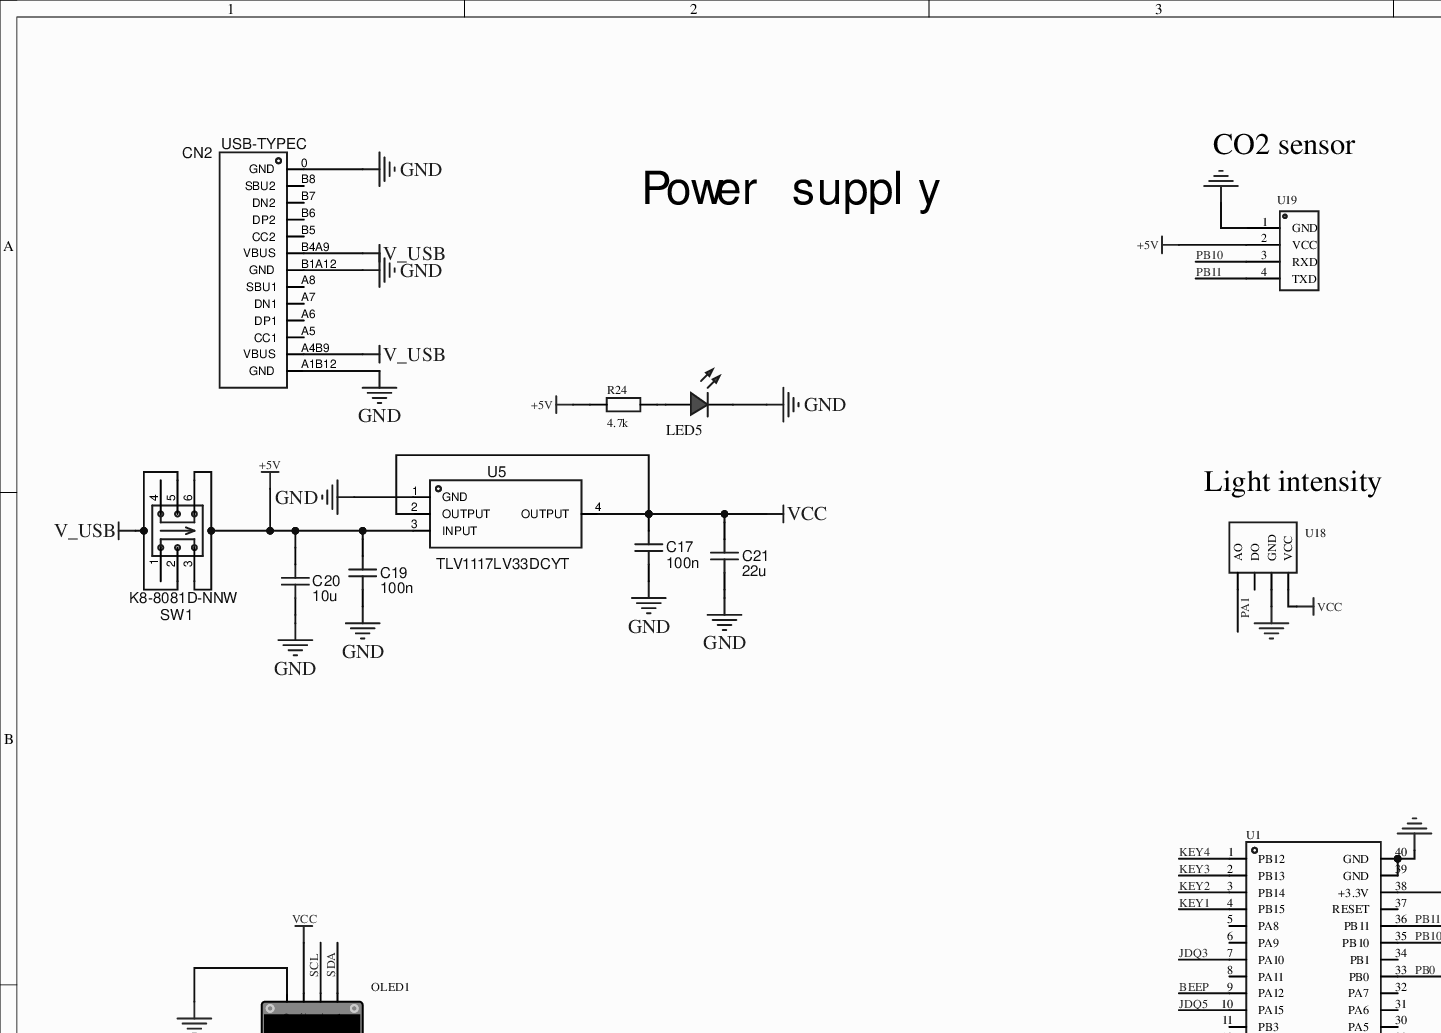
[diagram p0: MISC51965-3.schdoc, top left]
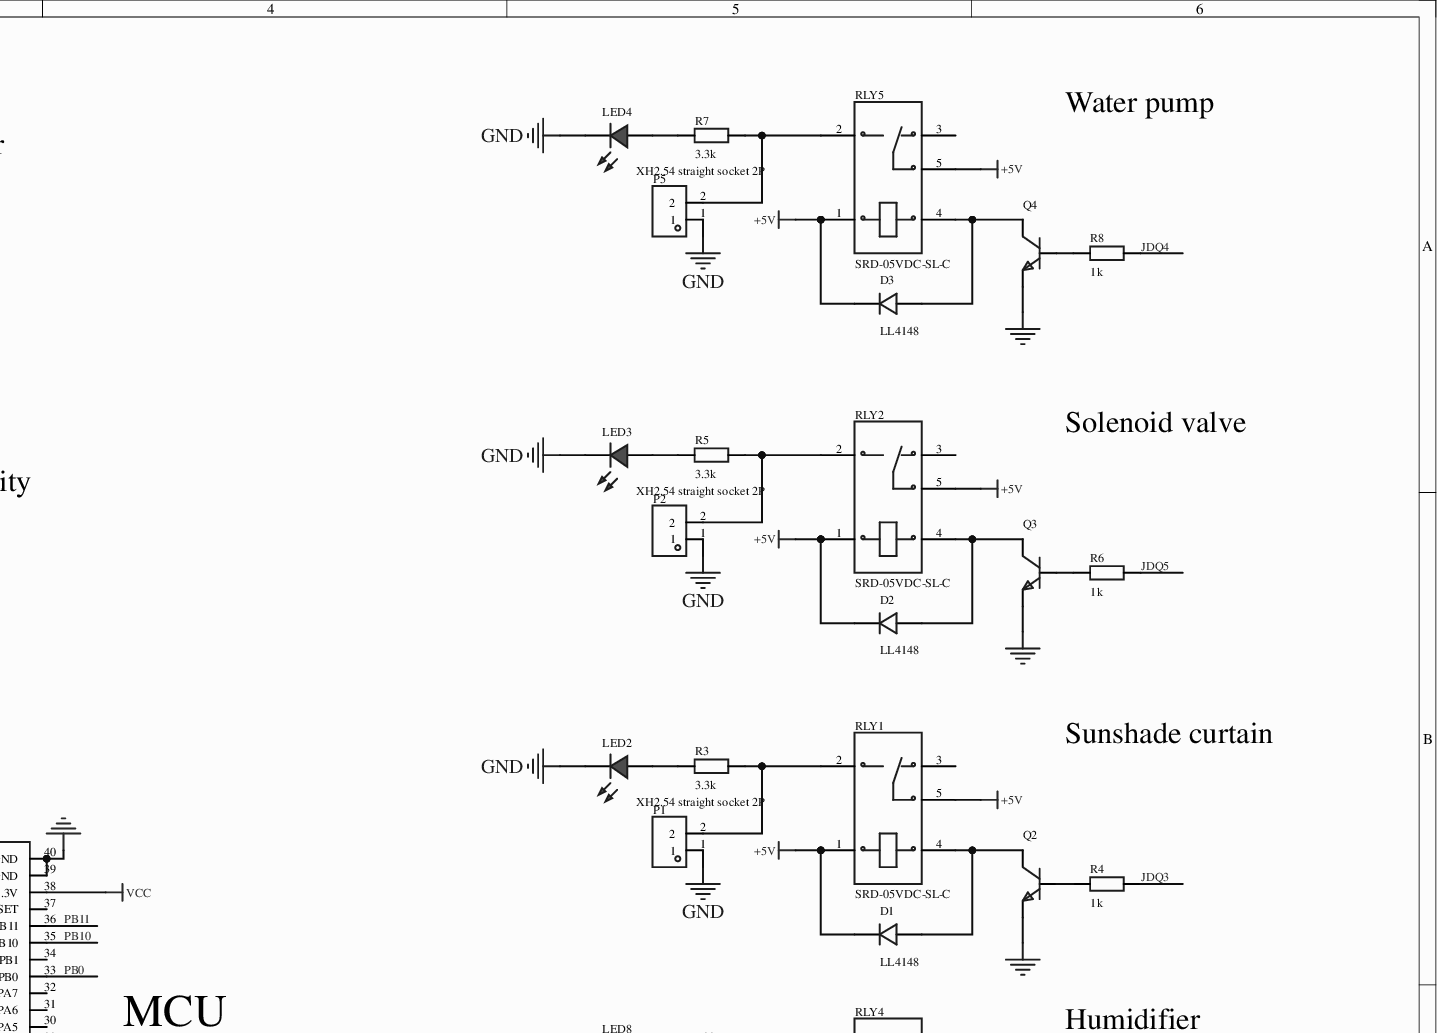
[diagram p1: MISC51965-3.schdoc, top right]
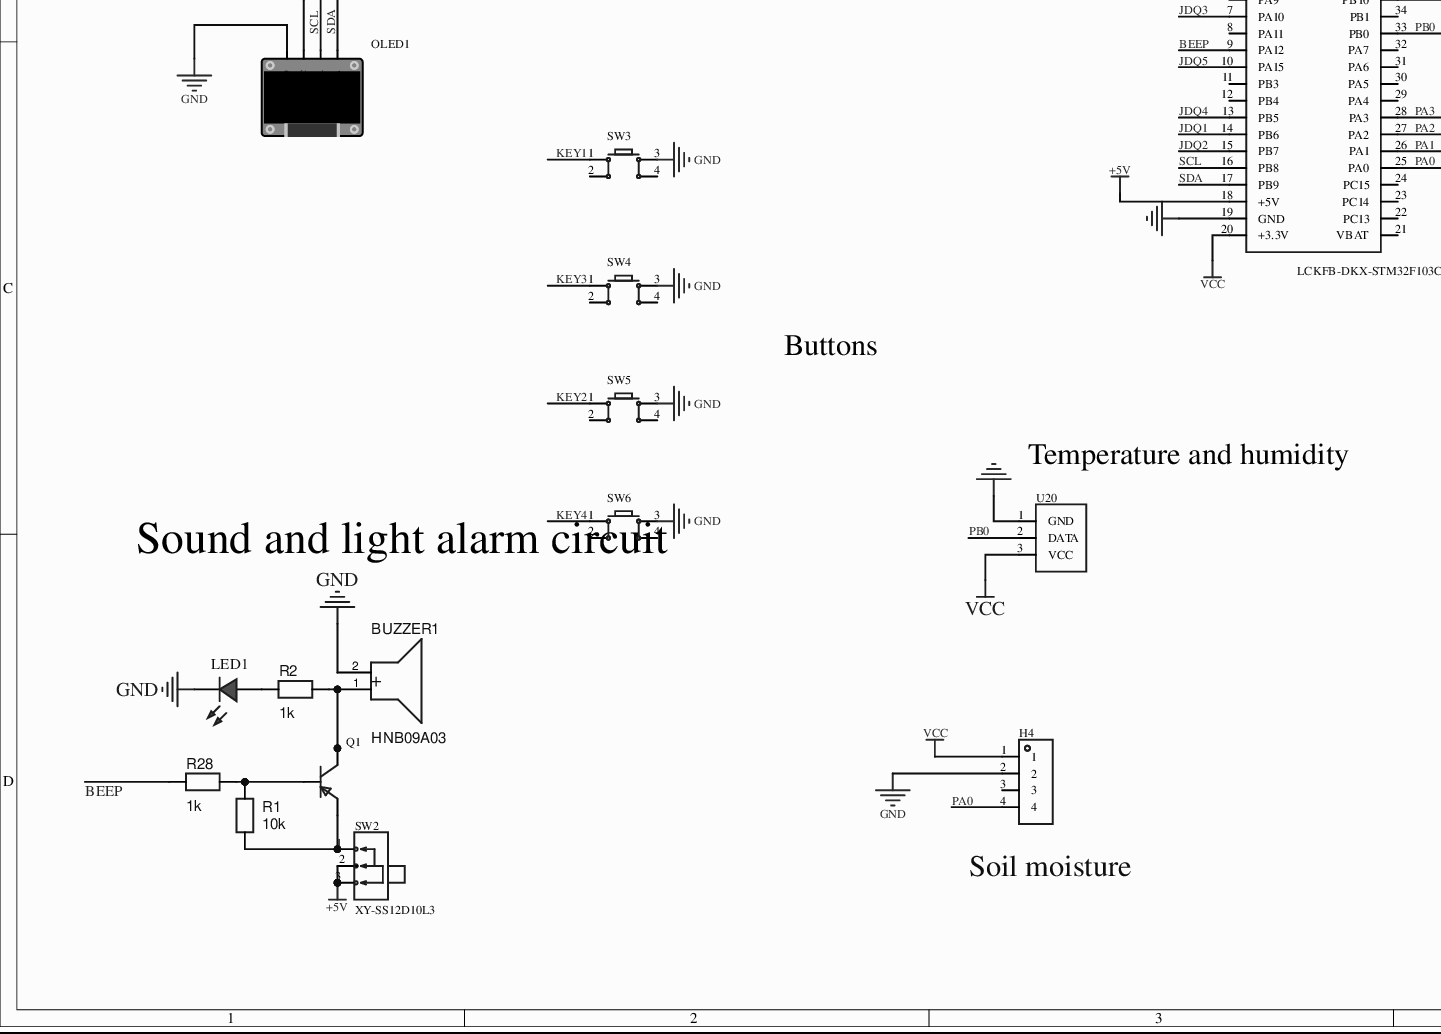
[diagram p2: MISC51965-3.schdoc, bottom left]
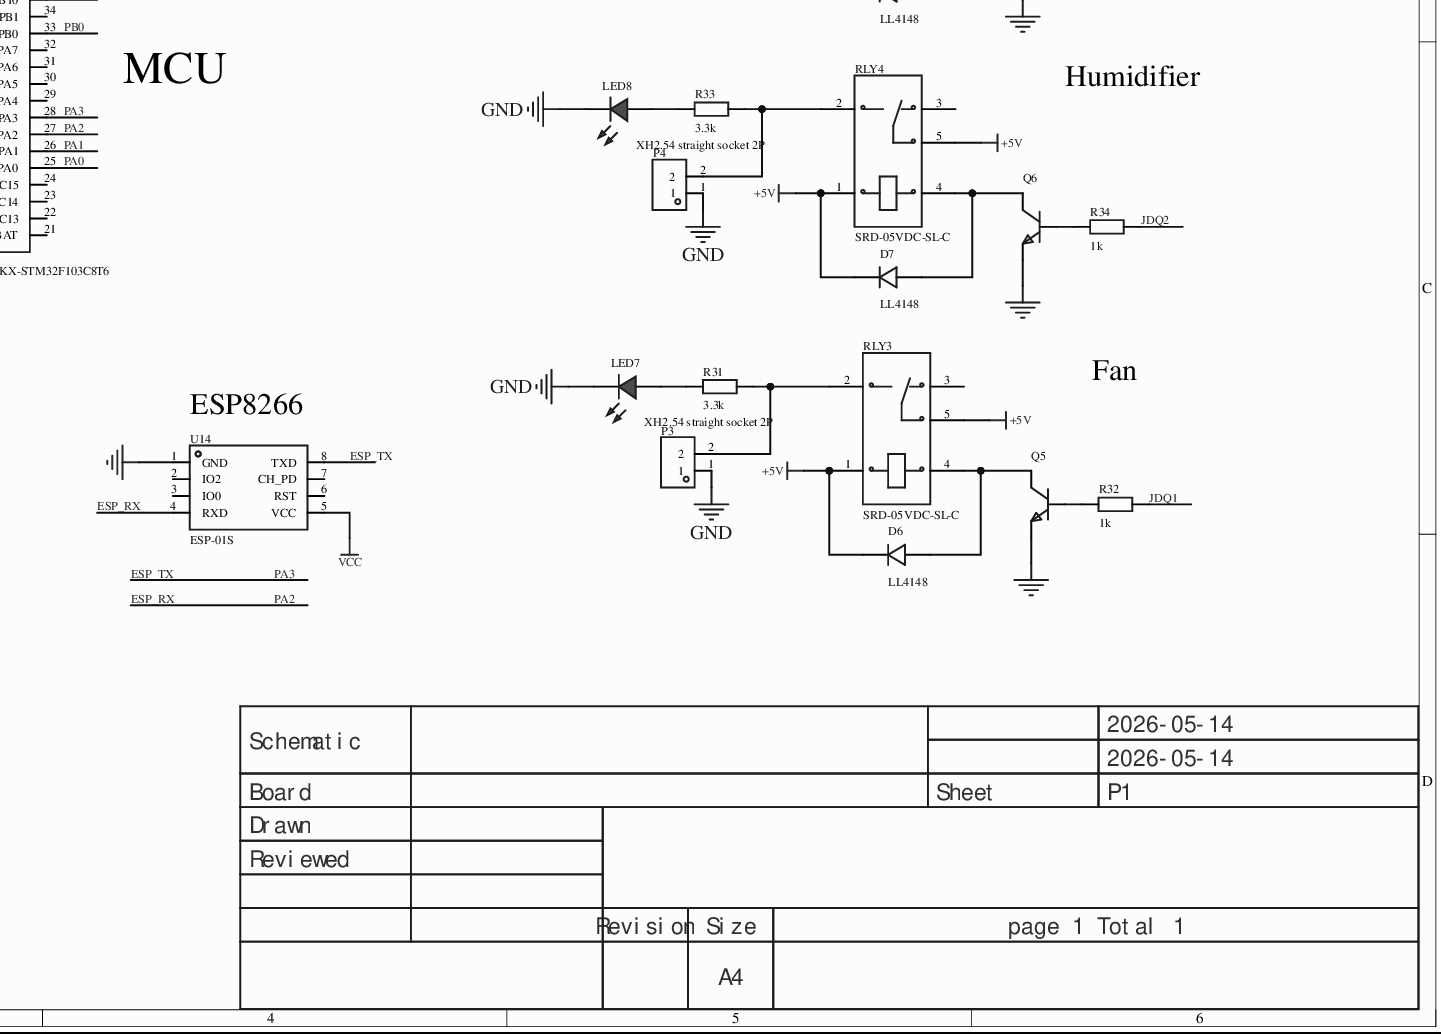
[diagram p3: MISC51965-3.schdoc, bottom right]
# Altium project MISC51965-2.PrjPcb
1 sheet, 62 parts. Net scope: global (net labels, ports and power ports of the same name join across sheets).
Board file: MISC51965.pcbdoc

## Sheet MISC51965-3.schdoc
size 420 x 297 mm; Version: V1.0; @Project Name: MISC51965; @Update Date: 2026-05-14; @Create Date: 2026-05-14; @Board Name: MISC51965; @Create Time: 12:43:51; @Page Count: 1; @Page No: 1; @Schematic Name: MISC51965; @Update Time: 12:43:51; Size: A4

### Parts
BUZZER1  HNB09A03  [BUZ-TH_BD9.0-P5.00-D0.6-FD]
C17  100n  [C0603]
C19  100n  [C0603]
C20  10u  [C0603]
C21  22u  [C0603]
CN2  USB-TYPEC  [USB-C-SMD_MC-307]
D1  LL4148  [LL-34_L3.5-W1.5-RD]
D2  LL4148  [LL-34_L3.5-W1.5-RD]
D3  LL4148  [LL-34_L3.5-W1.5-RD]
D6  LL4148  [LL-34_L3.5-W1.5-RD]
D7  LL4148  [LL-34_L3.5-W1.5-RD]
H4  (no value)  [HDR-TH_4P-P2.54-V-F]
LED1  (no value)  [LED_0603]
LED2  (no value)  [LED_TH-3mm]
LED3  (no value)  [LED_TH-3mm]
LED4  (no value)  [LED_TH-3mm]
LED5  (no value)  [LED_0603]
LED7  (no value)  [LED_TH-3mm]
LED8  (no value)  [LED_TH-3mm]
OLED1  (no value)  [0.96OLED_4P]
P1  XH2.54 straight socket 2P  [CONN-TH_XH2.54-2P]
P2  XH2.54 straight socket 2P  [CONN-TH_XH2.54-2P]
P3  XH2.54 straight socket 2P  [CONN-TH_XH2.54-2P]
P4  XH2.54 straight socket 2P  [CONN-TH_XH2.54-2P]
P5  XH2.54 straight socket 2P  [CONN-TH_XH2.54-2P]
Q1  (no value)  [S8550P_SOT]
Q2  (no value)  [S8050_SOT-23]
Q3  (no value)  [S8050_SOT-23]
Q4  (no value)  [S8050_SOT-23]
Q5  (no value)  [S8050_SOT-23]
Q6  (no value)  [S8050_SOT-23]
R1  10k  [R0603]
R2  1k  [R0603]
R3  3.3k  [R0603]
R4  1k  [R0603]
R5  3.3k  [R0603]
R6  1k  [R0603]
R7  3.3k  [R0603]
R8  1k  [R0603]
R24  4.7k  [R0805]
R28  1k  [R0603]
R31  3.3k  [R0603]
R32  1k  [R0603]
R33  3.3k  [R0603]
R34  1k  [R0603]
RLY1  SRD-05VDC-SL-C  [RELAY-TH_SRD-XXVDC-XL-C]
RLY2  SRD-05VDC-SL-C  [RELAY-TH_SRD-XXVDC-XL-C]
RLY3  SRD-05VDC-SL-C  [RELAY-TH_SRD-XXVDC-XL-C]
RLY4  SRD-05VDC-SL-C  [RELAY-TH_SRD-XXVDC-XL-C]
RLY5  SRD-05VDC-SL-C  [RELAY-TH_SRD-XXVDC-XL-C]
SW1  K8-8081D-NNW  [SW-TH_6P-L8.0-W8.0-P2.50]
SW2  XY-SS12D10L3  [SW-TH_3P-L12.7-W6.7_XY-SS12D10LXX]
SW3  (no value)  [SW-TH_4P-L6.0-W6.0-P4.50-LS6.5]
SW4  (no value)  [SW-TH_4P-L6.0-W6.0-P4.50-LS6.5]
SW5  (no value)  [SW-TH_4P-L6.0-W6.0-P4.50-LS6.5]
SW6  (no value)  [SW-TH_4P-L6.0-W6.0-P4.50-LS6.5]
U1  LCKFB-DKX-STM32F103C8T6  [CONN-TH_L53.3-W22.9_STM32F103C8T6-CARD]
U5  TLV1117LV33DCYT  [SOT-223-4_L6.5-W3.5-P2.30-LS7.0-BR]
U14  ESP-01S  [WIFIM-TH_ESP-01S]
U18  Light intensity module  [光敏传感器]  (value not drawn)
U19  (no value)  [4P排母]
U20  (no value)  [dht11温湿度传感器]

### Nets
+5V: C19.2 C20.2 D1.1(K) D2.1(K) D3.1(K) D6.1(K) D7.1(K) R24.1 RLY1.1 RLY1.5 RLY2.1 RLY2.5 RLY3.1 RLY3.5 RLY4.1 RLY4.5 RLY5.1 RLY5.5 SW1.3 SW1.6 SW2.2 SW2.3 U1.18(+5V) U5.3(INPUT) U19.2(VCC)
GND: BUZZER1.2(-) C17.1 C19.1 C20.1 C21.1 CN2.0(GND) CN2.A1B12(GND) CN2.B1A12(GND) H4.2 LED1.1(C) LED2.2(A) LED3.2(A) LED4.2(A) LED5.1(C) LED7.2(A) LED8.2(A) OLED1.1(GND) P1.1 P2.1 P3.1 P4.1 P5.1 Q2.2 Q3.2 Q4.2 Q5.2 Q6.2 SW3.3 SW4.3 SW5.3 SW6.3 U1.19(GND) U1.39(GND) U1.40(GND) U5.1(GND) U14.1(GND) U18.2(GND) U19.1(GND) U20.1(GND)
V_USB: CN2.A4B9(VBUS) CN2.B4A9(VBUS) SW1.2 SW1.5
VCC: C17.2 C21.2 H4.1 OLED1.2(VCC) U1.20(+3.3V) U1.38(+3.3V) U5.2(OUTPUT) U5.4(OUTPUT) U14.5(VCC) U18.1(VCC) U20.3(VCC)
BEEP: R28.1 U1.9(PA12)
ESP_RX: U1.27(PA2) U14.4(RXD)  [also labelled PA2]
ESP_TX: U1.28(PA3) U14.8(TXD)  [also labelled PA3]
JDQ1: R32.1 U1.14(PB6)
JDQ2: R34.1 U1.15(PB7)
JDQ3: R4.1 U1.7(PA10)
JDQ4: R8.1 U1.13(PB5)
JDQ5: R6.1 U1.10(PA15)
KEY1: SW3.1 U1.4(PB15)
KEY2: SW5.1 U1.3(PB14)
KEY3: SW4.1 U1.2(PB13)
KEY4: SW6.1 U1.1(PB12)
PA0: H4.4 U1.25(PA0)
PA1: U1.26(PA1) U18.4(AO)
PB0: U1.33(PB0) U20.2(DATA)
PB10: U1.35(PB10) U19.3(RXD)
PB11: U1.36(PB11) U19.4(TXD)
SCL: OLED1.3(SCL) U1.16(PB8)
SDA: OLED1.4(SDA) U1.17(PB9)
NetBUZZER1_1: BUZZER1.1(+) Q1.3(C) R2.2
NetD1_2: D1.2(A) Q2.3 RLY1.4
NetD2_2: D2.2(A) Q3.3 RLY2.4
NetD3_2: D3.2(A) Q4.3 RLY5.4
NetD6_2: D6.2(A) Q5.3 RLY3.4
NetD7_2: D7.2(A) Q6.3 RLY4.4
NetLED1_2: LED1.2(A) R2.1
NetLED2_1: LED2.1(C) R3.2
NetLED3_1: LED3.1(C) R5.2
NetLED4_1: LED4.1(C) R7.2
NetLED5_2: LED5.2(A) R24.2
NetLED7_1: LED7.1(C) R31.2
NetLED8_1: LED8.1(C) R33.2
NetP1_2: P1.2 R3.1 RLY1.2
NetP2_2: P2.2 R5.1 RLY2.2
NetP3_2: P3.2 R31.1 RLY3.2
NetP4_2: P4.2 R33.1 RLY4.2
NetP5_2: P5.2 R7.1 RLY5.2
NetQ1_1: Q1.1(B) R1.2 R28.2
NetQ1_2: Q1.2(E) R1.1 SW2.1
NetQ2_1: Q2.1 R4.2
NetQ3_1: Q3.1 R6.2
NetQ4_1: Q4.1 R8.2
NetQ5_1: Q5.1 R32.2
NetQ6_1: Q6.1 R34.2

Not connected (* = marked no-connect by the designer): CN2 A5(CC1)* A6(DP1) A7(DN1) A8(SBU1)* B5(CC2)* B6(DP2) B7(DN2) B8(SBU2)*; H4 3; RLY1 3*; RLY2 3*; RLY3 3*; RLY4 3*; RLY5 3*; SW1 1* 4*; SW3 2 4; SW4 2 4; SW5 2 4; SW6 2 4; U1 5(PA8) 6(PA9) 8(PA11) 11(PB3) 12(PB4) 21(VBAT) 22(PC13) 23(PC14) 24(PC15) 29(PA4) 30(PA5) 31(PA6) 32(PA7) 34(PB1) 37(RESET); U14 2(IO2)* 3(IO0)* 6(RST)* 7(CH_PD)*; U18 3(DO)*

### Notes on the sheet
- CO2 sensor
- Water pump
- Power supply
- Light intensity
- Solenoid valve
- Sunshade curtain
- MCU
- Humidifier
- Buttons
- Fan
- (near U20) Temperature and humidity
- (near U14) ESP8266
- (near SW6) Sound and light alarm circuit
- (near H4) Soil moisture
- 2026-05-14
- Schematic
- Board
- Sheet
- P1
- Drawn
- Reviewed
- Revision
- Size
- A4
- page 1 Total 1

### Library data of the parts
BUZZER1 = HNB09A03: Manufacturer: 华能; Add into BOM: yes; Frequency: 3kHz; Symbol: HNB09A03; Device: HNB09A03; Convert to PCB: yes; Origin Footprint: BUZ-TH_BD9.0-P5.00-D0.6-FD; Supplier: LCSC; Supplier Part: C96102; Manufacturer Part: HNB09A03; JLCPCB Part Class: Extended Part; FootprintName: BUZ-TH_BD9.0-P5.00-D0.6-FD
C17 C19-C21 = 100n: Add into BOM: yes; Symbol: 100n; Device: 100n; Convert to PCB: yes; Origin Footprint: C0603; FootprintName: C0603
CN2 = MC-307: Manufacturer: HANBO(汉博); Add into BOM: yes; Symbol: USB-TYPEC; Device: MC-307; Convert to PCB: yes; Origin Footprint: USB-C-SMD_MC-307; Supplier: LCSC; Supplier Part: C961709; Manufacturer Part: MC-307; JLCPCB Part Class: Extended Part; FootprintName: USB-C-SMD_MC-307
D1-D3 D6 D7 = LL4148_C9808: Diode configuration: -; power: 500mW; DC reverse withstand voltage (Vr): 75V; average rectified current (Io): 200mA; forward voltage (Vf): 1V@10mA; reverse current (Ir): 5uA@75V; reverse recovery time (trr): 4ns; operating temperature: +175℃@(Tj);; Manufacturer: ST(先科); 3D Model: 4a6f2309ca4c4217857da1816cccdf69; 3D Model Transform: 133.93674,59.031,0,0,0,0,0,0,0; AddInBom: yes; ModelName: LL-34_L3.5-W1.5; Symbol: LL4148; Device: LL4148_C9808; LCSC Part Name: 75V 200mA 4ns; Supplier Part: C9808; Manufacturer Part: LL4148; Supplier Footprint: LL-34; JLCPCB Part Class: Basic library; Datasheet: https://example.com/upload/public/pdf/source/20121108/1457706554347.pdf; Supplier: LCSC; Diode Configuration: -; Power Dissipation: 500mW; Reverse Voltage (Vr): 75V; Average Rectified Current (Io): 200mA; Forward Voltage (Vf@If): 1V@10mA; Reverse Leakage Current: 5uA@75V; Reverse Recovery Time (trr): 4ns; Operating Temperature: +175℃@(Tj); ConvertToPcb: yes; FootprintName: LL-34_L3.5-W1.5-RD
H4 = HDR-F_2.54_1x4P: Symbol: 2.54-1*4P female; 3D Model: d187812051054f85879fcaa51a310d8e0819f05c4eef4c71ace90d822a990e87; 3D Model Transform: 419.6842,98.464,0,0,0,0,0,0,-118.11; ConvertToPcb: yes; Device: HDR-F_2.54_1x4P; Supplier Part: C2718488; Supplier Footprint: 插件; FootprintName: HDR-TH_4P-P2.54-V-F; AddInBom: yes; ModelName: HDR-TH_4P-P2.54-V-F
LED1 LED5 = LED_0603-R: Symbol: LED_R; Convert to PCB: yes; 3D Model: dd8257b0d61a4cd7b68939a056e08095; 3D Model Transform: 58.72,29.4,22.03,0,0,0,0,0,0; ModelName: LED-0603_R; Device: LED_0603-R; Add into BOM: yes; Supplier Footprint: 0603; FootprintName: LED_0603
LED2-LED4 LED7 LED8 = LED_TH-R_3mm: 3D Model: a497c992633541038a38947cdc58012f; 3D Model Transform: 141.274,153.327,0,0,0,0,-5.984,0,-137.795; ConvertToPcb: yes; ModelName: LED-TH-3mm_R; Symbol: LED_TH-R; Device: LED_TH-R_3mm; Supplier Footprint: 插件; AddInBom: yes; FootprintName: LED_TH-3mm
OLED1 = 0.96OLED模块_4P: Symbol: 0.96OLED module_4P; ConvertToPcb: yes; ModelId: 79c000fdb68d45a296c2e9bedf4f90550819f05c4eef4c71ace90d822a990e87; ModelTransform: 1393.69792,1318.895,0,0,0,0,0,-560.079,-137.795; Device: 0.96OLED module_4P; AddInBom: yes; FootprintName: 0.96OLED_4P; Supplier Footprint: 插件; ModelName: 0.96OLED_4P
P1-P5 = XH2.54直插座-2P: 3D Model: dc9654a6caad4c20aab3bc231ea458cf; 3D Model Transform: 296.889,230.315,0,0,0,0,0,26.653,-137.795; AddInBom: yes; Symbol: XH2.54 straight socket 2P; Device: XH2.54 straight socket 2P; LCSC Part Name: XH2.54直插座-2P; Supplier Part: C9900016957; Manufacturer Part: XH2.54直插座-2P; Supplier Footprint: XH2.54-2; JLCPCB Part Class: Extended library; Supplier: LCSC; ConvertToPcb: yes; FootprintName: CONN-TH_XH2.54-2P; ModelName: CONN-TH_XH2.54-2P
Q1 = S8550_SOT_PNP: Symbol: PNP; ConvertToPcb: yes; ModelId: 9c0df02d6f3e44e889da37f3e5bf54960819f05c4eef4c71ace90d822a990e87; ModelName: SOT-23-3_L2.9-W1.4-P1.90-LS2.5-BR; ModelTransform: 98.43,114.17,37.91,0,0,0,0,0,0; Device: S8550_SOT_PNP; AddInBom: yes; Supplier Footprint: SOT-23; FootprintName: S8550P_SOT
Q2-Q6 = S8050_SOT_NPN: Symbol: NPN; 3D Model: c62791f0466c4ae2a892c056b845b0ca; 3D Model Transform: 98.6,114.12,41.29,180,0,0,0,0,-3; ConvertToPcb: yes; ModelName: SOT-23-3P_L2.9-W1.3-H1.0-LS2.4-P0.95; Device: S8050_SOT_NPN; Supplier Footprint: SOT-23; AddInBom: yes; FootprintName: S8050_SOT-23
R1 R2 R28 = 1k: Add into BOM: yes; Symbol: 1k; Device: 1k; Convert to PCB: yes; Origin Footprint: R0603; FootprintName: R0603
R3-R8 R31-R34 = Res_0603: Symbol: Resistor; 3D Model: fc143cca1e79419f9cd78b61e9279f08; 3D Model Transform: 31.8897,63.7794,0,90,0,0,0,0,0; ConvertToPcb: yes; Device: Res_0603; Supplier Footprint: 0603; AddInBom: yes; FootprintName: R0603; ModelName: R0603
  R3 R5 R7 R31 R33: Value: 3.3k
  R4 R6 R8 R32 R34: Value: 1k
R24 = 0805W8F1002T5E_C17414: Resistor type: thick film resistor; resistance: 10kΩ; tolerance: ±1%; power: 125mW;; Manufacturer: UNI-ROYAL(厚声); 3D Model: 37a81e68749a4138bd2dfa6897b24b85; 3D Model Transform: 78.74,51.181,0,0,0,0,0,-0.0005,0; Temperature Coefficient: ±100ppm/℃; Overload Voltage (Max): 150V; AddInBom: yes; ModelName: R0805_L2.0-W1.3-H0.6; Symbol: 0805W8F1002T5E; Device: 0805W8F1002T5E_C17414; Value: 4.7k; LCSC Part Name: 10kΩ ±1% 125mW; Manufacturer Part: 0805W8F1002T5E; Supplier Footprint: 0805; JLCPCB Part Class: Basic library; Datasheet: https://example.com/upload/public/pdf/source/20200306/C422600_1E6D84923E4A46A82E41ADD87F860B5C.pdf; Supplier: LCSC; Type: Thick film resistor; Tolerance: ±1%; Power(Watts): 125mW; Operating Temperature Range: -55℃~+155℃; ConvertToPcb: yes; FootprintName: R0805
RLY1-RLY5 = SRD-05VDC-SL-C: Coil voltage: 5V; contact form: 1C (SPDT changeover); contact rating (resistive load): -; max switching voltage: 250V@AC; max switching current: 15A;; Manufacturer: 松乐; 3D Model: d0eda9b8bf8746d18ae810ab88dc78e7; 3D Model Transform: 755.904,622.4397,0,0,0,0,34.882,0,-118.11; Pin Number: 5; Coil Rated Power: 360mW; Coil Type: Non-polar, single coil; Coil Resistance: 70Ω; Contact Resistance: 100mΩ; Operate Time: 10ms; AddInBom: yes; ModelName: RELAY-TH_L19.2-W15.6-H15.8; Symbol: SRD-05VDC-SL-C; Device: SRD-05VDC-SL-C; LCSC Part Name: 蓝色; Supplier Part: C35449; Manufacturer Part: SRD-05VDC-SL-C; Supplier Footprint: 插件,15.6x19.2mm; JLCPCB Part Class: Extended library; Datasheet: https://example.com/upload/public/pdf/source/20200305/C490149_C96E4098A3B1FFB377D5AD2E40B7C2A8.pdf; Supplier: LCSC; Coil Voltage: 5V; Contact Form: 1C (SPDT changeover); Contact Rating: -; Maximum Switching Voltage: 250V@AC; Maximum Switching Current: 15A; Release Time: 10ms; ConvertToPcb: yes; FootprintName: RELAY-TH_SRD-XXVDC-XL-C
SW1 = XKB8080-Z: Manufacturer: XKB Enterprise; Add into BOM: yes; Symbol: K8-8081D-NNW; Device: XKB8080-Z; Convert to PCB: yes; Origin Footprint: SW-TH_6P-L8.0-W8.0-P2.50; Supplier: LCSC; Supplier Part: C318860; Manufacturer Part: XKB8080-Z; FootprintName: SW-TH_6P-L8.0-W8.0-P2.50
SW2 = XY-SS12D10L3: Toggle switch, vertical straight pins, two-position, through-hole, single row, forward actuation, lever length 3mm; Manufacturer: XYECONN(辛译); AddInBom: yes; Symbol: XY-SS12D10L3; Device: XY-SS12D10L3; LCSC Part Name: 拨动开关,立式直脚两档,插件,单排正拨,柄长3mm; SupplierPart: C49652929; ManufacturerPart: XY-SS12D10L3; Supplier Footprint: 插件; JLCPCB Part Class: Extended Part; Datasheet: https://example.com/datasheet/XY-SS12D10L3/52215304.html; Supplier: LCSC; ConvertToPcb: yes; FootprintName: SW-TH_3P-L12.7-W6.7_XY-SS12D10LXX
SW3-SW6 = Key_TH_6x6x6: Contact current: 50mA; rated voltage (DC): 12V; insulation resistance: 100MΩ; circuit structure: SPST; mounting: through-hole; button shape: round; button/cap color: black; actuating force: 260gf@±30gf; operating temperature: -25℃~+70℃; pin style: PC pin; switch length: 6mm; switch width: 6mm; switch height: 6mm; with bracket: no;; Symbol: Tactile switch; AddInBom: yes; ModelId: 20eee248bc684ccd8cbdbb1d0d91ec6f0819f05c4eef4c71ace90d822a990e87; ModelName: SW-TH_4P-L6.0-W6.0-H5.0-LS6.5-P4.50; ModelTransform: 236.22,323.03,0,90,0,0,0,0,-137.795; Device: Key_TH_6x6x6; ConvertToPcb: yes; FootprintName: SW-TH_4P-L6.0-W6.0-P4.50-LS6.5; Supplier Footprint: 插件
U1 = LCKFB-DKX-STM32F103C8T6: Manufacturer: 立创开发板; AddInBom: yes; Symbol: LCKFB-DKX-STM32F103C8T6; Device: LCKFB-DKX-STM32F103C8T6; LCSC Part Name: 立创·地阔星-STM32F103C8T6开发板; Supplier Part: C22396880; Manufacturer Part: LCKFB-DKX-STM32F103C8T6; Supplier Footprint: -; JLCPCB Part Class: Extended library; Datasheet: https://example.com/upload/public/pdf/source/20240801/7EEF69F7480DF7C6DA98696664D658D4.pdf; Supplier: LCSC; ConvertToPcb: yes; FootprintName: CONN-TH_L53.3-W22.9_STM32F103C8T6-CARD
U5 = TLV1117LV33DCYT: Manufacturer: TI(德州仪器); Add into BOM: yes; Symbol: TLV1117LV33DCYT; Device: TLV1117LV33DCYT; Convert to PCB: yes; Origin Footprint: SOT-223-4_L6.5-W3.5-P2.30-LS7.0-BR; Supplier: LCSC; Supplier Part: C2877977; Manufacturer Part: TLV1117LV33DCYT; JLCPCB Part Class: Extended Part; FootprintName: SOT-223-4_L6.5-W3.5-P2.30-LS7.0-BR
U14 = ESP-01S_C111009: 3D Model: eb7175da78ae48b3b1568cfe3027405f; 3D Model Transform: 582.676,976.37608,0,0,0,0,0,388.346,-118.11; AddInBom: yes; Symbol: ESP-01S; Device: ESP-01S_C111009; LCSC Part Name: ESP-01S; Supplier Part: C111009; Manufacturer Part: ESP-01S; Supplier Footprint: -; Supplier: LCSC; ConvertToPcb: yes; FootprintName: WIFIM-TH_ESP-01S; ModelName: WIFIM-TH_ESP-01S
U18 = 光照强度模块: ConvertToPcb: yes; Symbol: Light intensity module; Device: Light intensity module; Supplier Part: C115245; Supplier: LCSC; AddInBom: yes; FootprintName: Photosensitive sensor
U19 = 二氧化碳传感器: Symbol: CO2 sensor; AddInBom: yes; Device: CO2 sensor; ConvertToPcb: yes; FootprintName: 4P female header
U20 = DHT11: AddInBom: yes; Symbol: DHT11; Device: DHT11; ConvertToPcb: yes; FootprintName: DHT11 temperature and humidity sensor